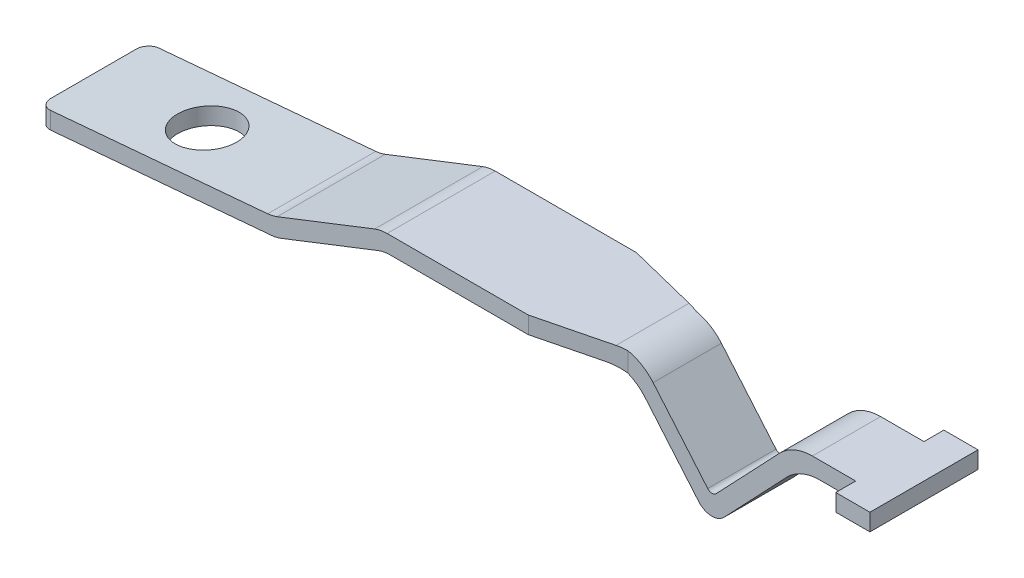
SolidWorks part; units mm, degrees
ref_plane "Front Plane" through (0, 0, 0) normal (0, 0, 1) x (1, 0, 0)
ref_plane "Top Plane" through (0, 0, 0) normal (0, 1, 0) x (1, 0, 0)
ref_plane "Right Plane" through (0, 0, 0) normal (1, 0, 0) x (0, 0, -1)
sketch "Sketch1" plane through (0, 0, 0) normal (0, 0, 1) x (1, 0, 0)
  line L0 (128.4721, 20.626) -> (135.2795, 20.626)
  line L1 (62.4102, 13.626) -> (82.6957, 15.4008)
  line L2 (83.5261, 15.5951) -> (92.0356, 18.9203)
  line L3 (93.1275, 19.126) -> (110.7311, 19.126)
  line L5 (113.7827, 17.712) -> (118.4908, 12.1563)
  line L6 (120.7231, 12.0934) -> (126.2152, 17.8797)
  line L7 (62.4102, 13.626) -> (2453.4899, 13.626) construction
  line L8 (135.2795, 19.126) -> (135.2795, 20.626)
  line L9 (62.2795, 15.1203) -> (82.3504, 16.8763)
  line L10 (83.1808, 17.0706) -> (91.753, 20.4203)
  line L11 (92.8448, 20.626) -> (111.4261, 20.626)
  line L12 (115.0486, 16.2182) -> (119.5719, 10.8805) construction
  line L13 (114.4777, 19.212) -> (119.2748, 13.5513)
  line L14 (120.0189, 13.5303) -> (125.5709, 19.3797)
  line L15 (62.4102, 13.626) -> (62.2795, 15.1203)
  line L16 (59.7583, 14.8997) -> (82.7795, 16.9138) construction
  line L17 (66.8652, 4.2394) -> (59.7583, 14.8997) construction
  line L18 (68.1133, 5.0715) -> (62.4102, 13.626) construction
  line L19 (82.7795, 16.9138) -> (92.2795, 20.626) construction
  line L20 (92.2795, 20.626) -> (111.1033, 20.626) construction
  line L21 (92.5622, 19.126) -> (110.6521, 19.126) construction
  line L22 (83.1248, 15.4383) -> (92.5622, 19.126) construction
  line L23 (62.4102, 13.626) -> (83.1248, 15.4383) construction
  line L24 (62.2795, 15.1203) -> (82.7795, 16.9138) construction
  line L25 (119.6351, 13.126) -> (126.7538, 20.626) construction
  line L26 (126.7538, 20.626) -> (135.2795, 20.626) construction
  line L27 (116.0546, 17.3513) -> (119.6351, 13.126) construction
  line L31 (129.1165, 19.126) -> (135.2795, 19.126)
  line L32 (129.2671, 19.126) -> (135.2795, 19.126) construction
  line L33 (119.5719, 10.8805) -> (127.8418, 19.5934) construction
  line L34 (129.2671, 19.126) -> (129.2671, 19.126) construction
  line L35 (129.2671, 19.126) -> (129.2671, 19.126) construction
  line L36 (129.2671, 19.126) -> (129.2671, 19.126) construction
  line L37 (129.2671, 19.126) -> (129.2671, 19.126) construction
  line L38 (129.2671, 19.126) -> (129.2671, 19.126) construction
  line L39 (129.2671, 19.126) -> (129.2671, 19.126) construction
  line L40 (129.2671, 19.126) -> (129.2671, 19.126) construction
  line L41 (129.2671, 19.126) -> (129.2671, 19.126) construction
  line L42 (129.2671, 19.126) -> (129.2671, 19.126) construction
  line L43 (129.2671, 19.126) -> (129.2671, 19.126) construction
  line L44 (129.2671, 19.126) -> (129.2671, 19.126) construction
  line L45 (129.2671, 19.126) -> (129.2671, 19.126) construction
  line L46 (129.2671, 19.126) -> (129.2671, 19.126) construction
  line L47 (110.6521, 19.126) -> (115.0486, 16.2182) construction
  line L48 (111.1033, 20.626) -> (116.0546, 17.3513) construction
  arc A0 (91.753, 20.4203) -> (92.8448, 20.626) centre (92.8448, 17.626) cw
  arc A1 (93.1275, 19.126) -> (92.0356, 18.9203) centre (93.1275, 16.126) ccw
  arc A2 (82.6957, 15.4008) -> (83.5261, 15.5951) centre (82.4342, 18.3893) ccw
  arc A3 (83.1808, 17.0706) -> (82.3504, 16.8763) centre (82.0889, 19.8649) cw
  arc A4 (125.5709, 19.3797) -> (128.4721, 20.626) centre (128.4721, 16.626) cw
  arc A5 (129.1165, 19.126) -> (126.2152, 17.8797) centre (129.1165, 15.126) ccw
  arc A6 (111.4261, 20.626) -> (114.4777, 19.212) centre (111.4261, 16.626) cw
  arc A7 (113.7827, 17.712) -> (110.7311, 19.126) centre (110.7311, 15.126) ccw
  arc A8 (120.7231, 12.0934) -> (118.4908, 12.1563) centre (119.6351, 13.126) cw
  arc A9 (119.2748, 13.5513) -> (120.0189, 13.5303) centre (119.6562, 13.8745) ccw
  point P38 (92.2795, 20.626)
  point P55 (113.2795, 20.626)
  dimension "D12" = 3
  dimension "D13" = 4
  dimension "D7" = 4
  dimension "D9" = 1.5
  dimension "D10" = 0.5
  dimension "D1" = 5
  dimension "D3" = 7
  dimension "D4" = 0
  dimension "D5" = 30
  dimension "D6" = 21
  dimension "D11" = 73
  dimension "D14" = 7.5
  dimension "D2" = 1.5
  dimension "D8" = 1.5
extrude "Boss-Extrude1" add sketch "Sketch1" along normal mid plane 9.5
sketch "Sketch2" plane through (0, 0, 0) normal (0, 1, 0) x (1, 0, 0)
  line L0 (59.0832, 0) -> (138.7471, 0) construction
  line L1 (132.2795, 4.75) -> (132.2795, 3)
  line L2 (63.2795, 4.75) -> (105.2569, 4.75)
  line L3 (62.2795, 3.75) -> (62.2795, -3.75)
  line L4 (63.2795, -4.75) -> (105.2569, -4.75)
  line L5 (135.2795, 4.75) -> (135.2795, -4.75)
  line L6 (112.2569, 3) -> (132.2795, 3)
  line L7 (112.2569, -3) -> (132.2795, -3)
  line L8 (132.2795, -3) -> (132.2795, -4.75)
  line L9 (110.7311, -4.75) -> (113.7827, -4.75) construction
  line L10 (112.2569, 3) -> (105.2569, 4.75)
  line L11 (112.2569, -3) -> (105.2569, -4.75)
  line L12 (132.2795, 4.75) -> (135.2795, 4.75)
  line L13 (132.2795, -4.75) -> (135.2795, -4.75)
  circle A0 centre (72.2795, 0) radius 2.6
  arc A1 (63.2795, -4.75) -> (62.2795, -3.75) centre (63.2795, -3.75) cw
  arc A2 (63.2795, 4.75) -> (62.2795, 3.75) centre (63.2795, 3.75) ccw
  point P16 (112.2569, -4.75)
  point P26 (62.2795, 4.75)
  dimension "D8" = 5.2
  dimension "D10" = 1
  dimension "D1" = 3
  dimension "D2" = 3
  dimension "D3" = 3
  dimension "D4" = 7
  dimension "D5" = 7
  dimension "D6" = 0
  dimension "D7" = 0
  dimension "D9" = 10
extrude "Cut-Extrude1" cut sketch "Sketch2" along normal blind 30 flip side to cut
